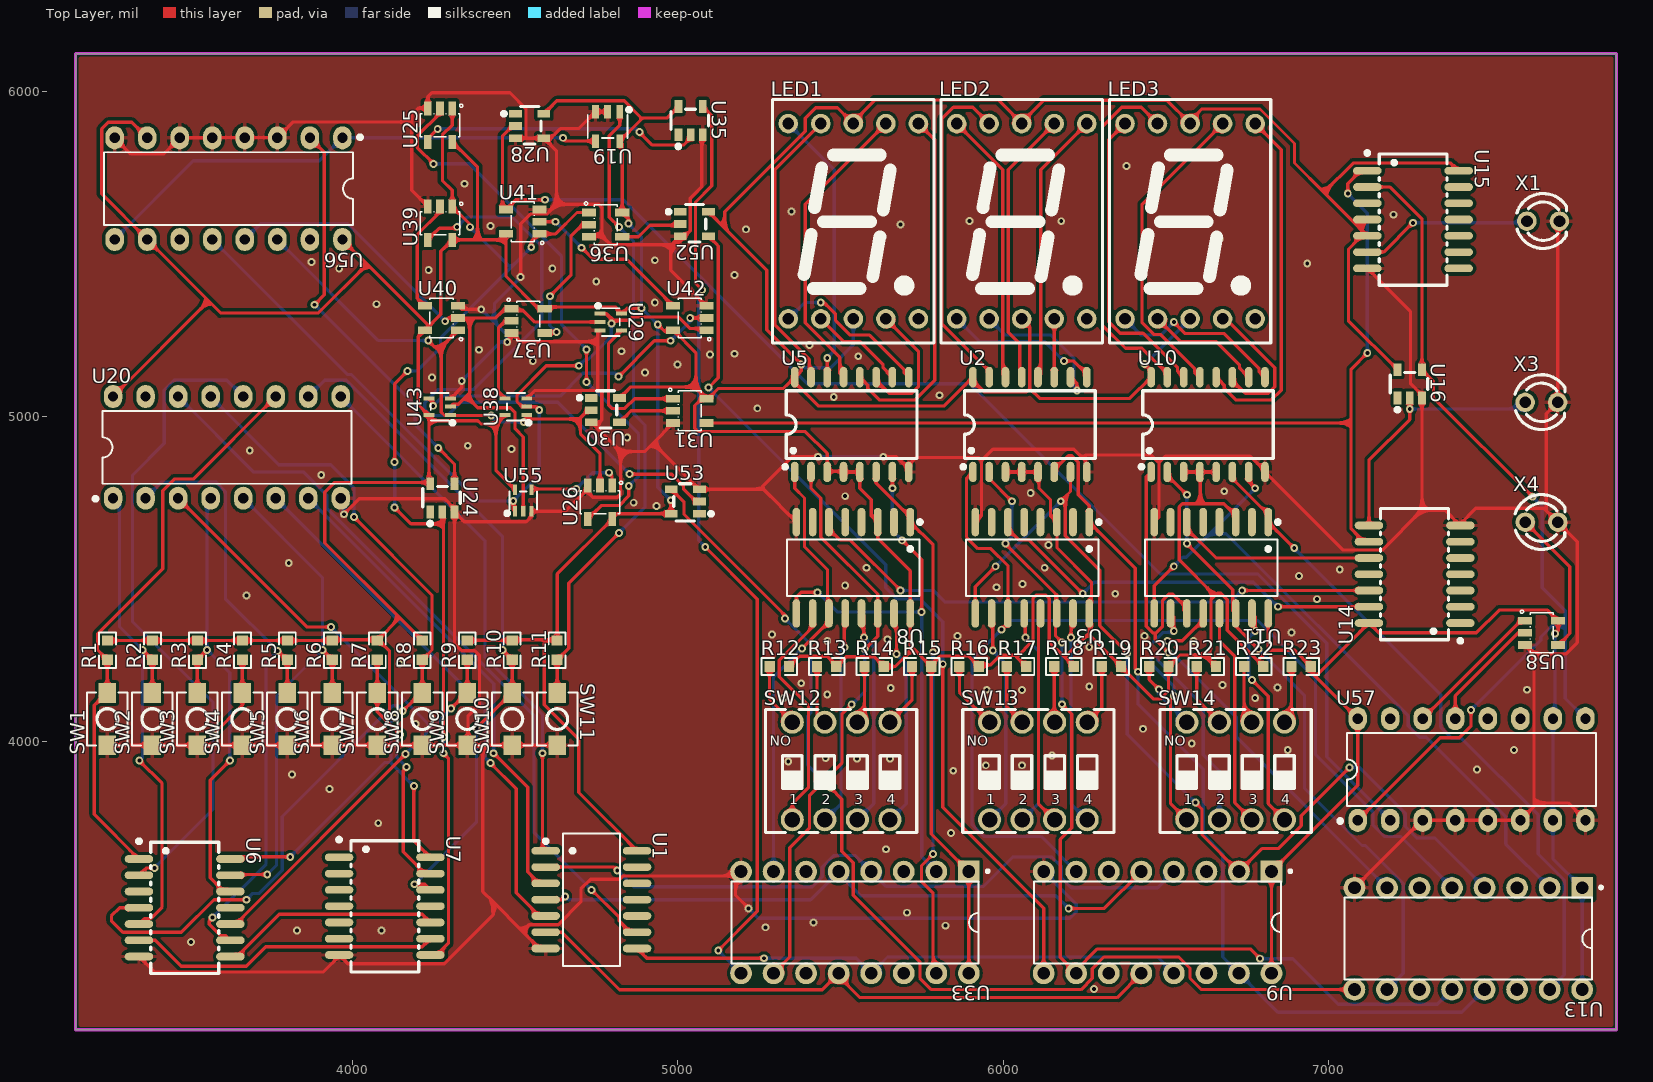
[diagram p0: Top Layer view]
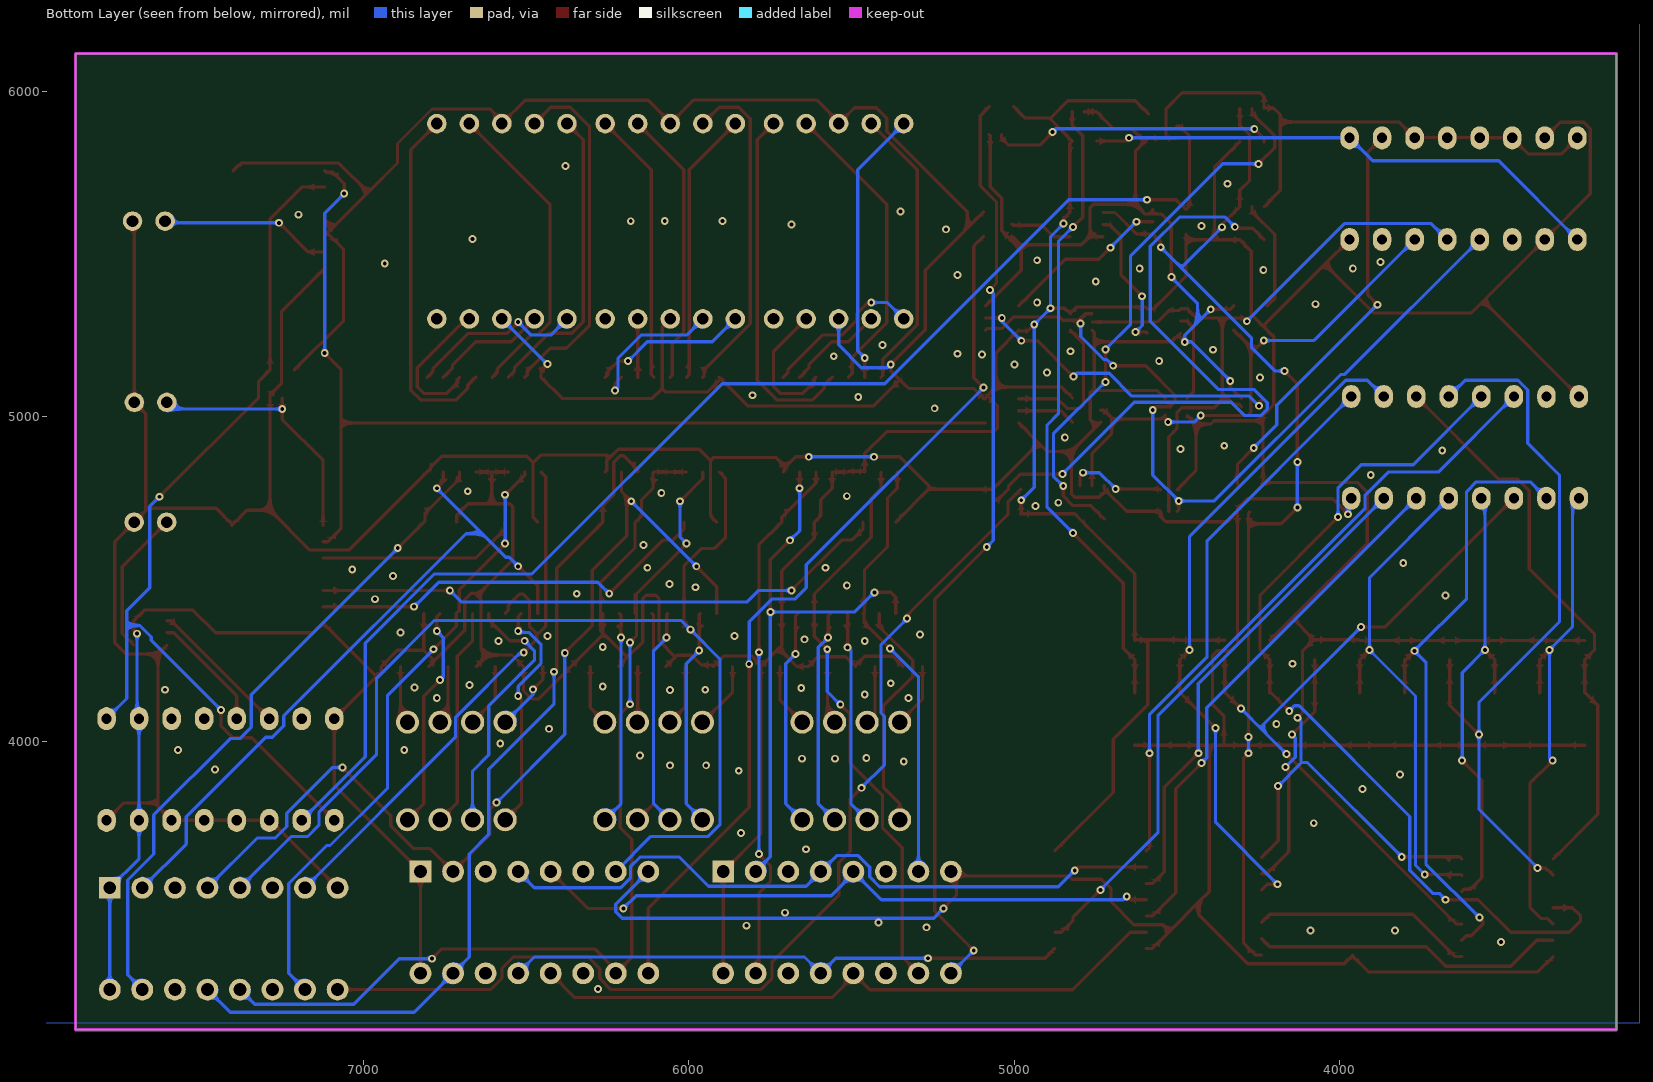
[diagram p1: Bottom Layer view, seen from below]
# Altium PCB MISC50897.pcbdoc (part 1 of 2)
Units mil, origin at the board's own origin, x right, y up, seen from the top; angles counter-clockwise.
Board outline 4735 x 3000 mil, 2 copper layers (Top Layer, Bottom Layer), stack 62.206 mil thick; 82 components, 112 nets, 500 pads, 251 vias.

## Layer stack, top to bottom
Top Solder Mask Layer: solder mask 0.394, Dk 3.3
Top Layer: signal copper 1.379
Dielectric1: surface 59.449, FR4, Dk 4.5
Bottom Layer: signal copper 1.378
Bottom Solder Mask Layer: solder mask 0.394, Dk 3.3

## Board outline
3150,6115 3150,3115 7885,3115 7885,6115

## Design rules (kind name [scope] priority, off if disabled: settings)
BoardOutlineClearance copperThickness2oz_1 [All] p2 off: genericclearance=7.99 ignorepadtopadclearanceinfootprint=FALSE except(0: Arc-SplitContinuation Track-SplitContinuation SMDPad-SplitContinuation THPad-SplitContinuation Via-SplitContinuation Fill-SplitContinuation Region-SplitContinuation Poly-SplitContinuation Text-SplitContinuation Hole-SplitContinuation; 5.98: Arc-CutoutEdge Track-CutoutEdge SMDPad-CutoutEdge THPad-CutoutEdge Via-CutoutEdge Text-CutoutEdge; 6.9: Hole-OutlineEdge Hole-CutoutEdge; 10: Poly-OutlineEdge Poly-CutoutEdge; 11.81: Arc-OutlineEdge Track-OutlineEdge SMDPad-OutlineEdge THPad-OutlineEdge Via-OutlineEdge Fill-OutlineEdge Region-OutlineEdge Text-OutlineEdge Fill-CutoutEdge Region-CutoutEdge)
BoardOutlineClearance Plane_innerPlane_1 [All] p4 off: genericclearance=4.02 ignorepadtopadclearanceinfootprint=FALSE except(0: Arc-SplitContinuation Track-SplitContinuation SMDPad-SplitContinuation THPad-SplitContinuation Via-SplitContinuation Fill-SplitContinuation Region-SplitContinuation Poly-SplitContinuation Text-SplitContinuation Hole-SplitContinuation; 5.98: Arc-CutoutEdge Track-CutoutEdge SMDPad-CutoutEdge THPad-CutoutEdge Via-CutoutEdge Text-CutoutEdge; 6.9: Hole-OutlineEdge Hole-CutoutEdge; 10: Poly-OutlineEdge Poly-CutoutEdge; 11.81: Arc-OutlineEdge Track-OutlineEdge SMDPad-OutlineEdge THPad-OutlineEdge Via-OutlineEdge Fill-OutlineEdge Region-OutlineEdge Text-OutlineEdge Fill-CutoutEdge Region-CutoutEdge)
BoardOutlineClearance Copper_copperRegion_1 [All] p6 off: genericclearance=4.02 ignorepadtopadclearanceinfootprint=FALSE except(0: Arc-SplitContinuation Track-SplitContinuation SMDPad-SplitContinuation THPad-SplitContinuation Via-SplitContinuation Fill-SplitContinuation Region-SplitContinuation Poly-SplitContinuation Text-SplitContinuation Hole-SplitContinuation; 5.98: Arc-CutoutEdge Track-CutoutEdge SMDPad-CutoutEdge THPad-CutoutEdge Via-CutoutEdge Text-CutoutEdge; 6.9: Hole-OutlineEdge Hole-CutoutEdge; 10: Poly-OutlineEdge Poly-CutoutEdge; 11.81: Arc-OutlineEdge Track-OutlineEdge SMDPad-OutlineEdge THPad-OutlineEdge Via-OutlineEdge Fill-OutlineEdge Region-OutlineEdge Text-OutlineEdge Fill-CutoutEdge Region-CutoutEdge)
BoardOutlineClearance copperThickness1oz_1 [All] p8: genericclearance=4.02 ignorepadtopadclearanceinfootprint=FALSE except(0: Arc-SplitContinuation Track-SplitContinuation SMDPad-SplitContinuation THPad-SplitContinuation Via-SplitContinuation Fill-SplitContinuation Region-SplitContinuation Poly-SplitContinuation Text-SplitContinuation Hole-SplitContinuation; 5.98: Arc-CutoutEdge Track-CutoutEdge SMDPad-CutoutEdge THPad-CutoutEdge Via-CutoutEdge Text-CutoutEdge; 6.9: Hole-OutlineEdge Hole-CutoutEdge; 10: Poly-OutlineEdge Poly-CutoutEdge; 11.81: Arc-OutlineEdge Track-OutlineEdge SMDPad-OutlineEdge THPad-OutlineEdge Via-OutlineEdge Fill-OutlineEdge Region-OutlineEdge Text-OutlineEdge Fill-CutoutEdge Region-CutoutEdge)
Clearance copperThickness2oz [All] p1 off: gap=7.99 ignorepadtopadclearanceinfootprint=FALSE except(5.98: SMDPad-Track SMDPad-SMDPad THPad-Track SMDPad-THPad THPad-THPad Track-Via SMDPad-Via THPad-Via Via-Via Fill-SMDPad Region-SMDPad Fill-THPad Region-THPad Fill-Via Region-Via Fill-Fill Fill-Region Region-Region Arc-Track Arc-SMDPad Arc-THPad Arc-Via Fill-Arc Region-Arc Arc-Arc Text-Track SMDPad-Text Text-THPad Text-Via Fill-Text Region-Text Arc-Text Text-Text; 6.9: Hole-Track Hole-SMDPad Hole-THPad Hole-Via Fill-Hole Region-Hole Hole-Arc Hole-Text; 10: Poly-Track Poly-SMDPad Poly-THPad Poly-Via Poly-Fill Poly-Region Poly-Poly Poly-Arc Poly-Text Poly-Hole; 11.81: Fill-Track Region-Track)
Clearance Plane_innerPlane [All] p3 off: gap=4.02 ignorepadtopadclearanceinfootprint=FALSE except(5.98: SMDPad-Track SMDPad-SMDPad THPad-Track SMDPad-THPad THPad-THPad Track-Via SMDPad-Via THPad-Via Via-Via Fill-SMDPad Region-SMDPad Fill-THPad Region-THPad Fill-Via Region-Via Fill-Fill Fill-Region Region-Region Arc-Track Arc-SMDPad Arc-THPad Arc-Via Fill-Arc Region-Arc Arc-Arc Text-Track SMDPad-Text Text-THPad Text-Via Fill-Text Region-Text Arc-Text Text-Text; 6.9: Hole-Track Hole-SMDPad Hole-THPad Hole-Via Fill-Hole Region-Hole Hole-Arc Hole-Text; 10: Poly-Track Poly-SMDPad Poly-THPad Poly-Via Poly-Fill Poly-Region Poly-Poly Poly-Arc Poly-Text Poly-Hole; 11.81: Fill-Track Region-Track)
Clearance Copper_copperRegion [All] p5 off: gap=4.02 ignorepadtopadclearanceinfootprint=FALSE except(5.98: SMDPad-Track SMDPad-SMDPad THPad-Track SMDPad-THPad THPad-THPad Track-Via SMDPad-Via THPad-Via Via-Via Fill-SMDPad Region-SMDPad Fill-THPad Region-THPad Fill-Via Region-Via Fill-Fill Fill-Region Region-Region Arc-Track Arc-SMDPad Arc-THPad Arc-Via Fill-Arc Region-Arc Arc-Arc Text-Track SMDPad-Text Text-THPad Text-Via Fill-Text Region-Text Arc-Text Text-Text; 6.9: Hole-Track Hole-SMDPad Hole-THPad Hole-Via Fill-Hole Region-Hole Hole-Arc Hole-Text; 10: Poly-Track Poly-SMDPad Poly-THPad Poly-Via Poly-Fill Poly-Region Poly-Poly Poly-Arc Poly-Text Poly-Hole; 11.81: Fill-Track Region-Track)
Clearance copperThickness1oz [All] p7: gap=4.02 ignorepadtopadclearanceinfootprint=FALSE except(5.98: SMDPad-Track SMDPad-SMDPad THPad-Track SMDPad-THPad THPad-THPad Track-Via SMDPad-Via THPad-Via Via-Via Fill-SMDPad Region-SMDPad Fill-THPad Region-THPad Fill-Via Region-Via Fill-Fill Fill-Region Region-Region Arc-Track Arc-SMDPad Arc-THPad Arc-Via Fill-Arc Region-Arc Arc-Arc Text-Track SMDPad-Text Text-THPad Text-Via Fill-Text Region-Text Arc-Text Text-Text; 6.9: Hole-Track Hole-SMDPad Hole-THPad Hole-Via Fill-Hole Region-Hole Hole-Arc Hole-Text; 10: Poly-Track Poly-SMDPad Poly-THPad Poly-Via Poly-Fill Poly-Region Poly-Poly Poly-Arc Poly-Text Poly-Hole; 11.81: Fill-Track Region-Track)
DiffPairsRouting differentialPair [All] p1: maxlimit=6 minlimit=6 mostfreqgap=6 toplayer_minwidth=5 toplayer_prefwidth=10 toplayer_maxwidth=100 toplayer_mingap=6 toplayer_prefgap=6 toplayer_maxgap=6 bottomlayer_minwidth=5 bottomlayer_prefwidth=10 bottomlayer_maxwidth=100 bottomlayer_mingap=6 bottomlayer_prefgap=6 bottomlayer_maxgap=6 maxuncoupledlength=10
HoleToHoleClearance otherClearance [All] p1: gap=11.81 allowstackedmicrovias=TRUE
Length netLength [All] p1: minlimit=0 maxlimit=0
PasteMaskExpansion pasteMaskExpansion [All] p1: expansion=0
PlaneConnect innerPlane [All] p1: planeconnectstyle=Relief reliefexpansion=20 reliefentries=4 reliefconductorwidth=10 reliefairgap=10
PolygonConnect copperRegion [All] p1: connectstyle=Relief reliefconductorwidth=10 reliefentries=4 polygonreliefangle="90 Angle" airgapwidth=10 via.connectstyle=Relief via.reliefconductorwidth=10 via.reliefentries=4 via.polygonreliefangle="90 Angle" via.airgapwidth=10
RoutingVias viaSize [All] p1: holewidth=12.01 width=24.02 viastyle="Through Hole" minholewidth=11.81 minwidth=19.68 maxholewidth=248.03 maxwidth=393.7
SolderMaskExpansion solderMaskExpansion [IsVia] p1: expansion=-1000 istentingtop=TRUE
SolderMaskExpansion solderMaskExpansion [All] p2: expansion=2 istentingtop=FALSE
Width copperThickness2oz_2 [All] p1 off: maxlimit=100 minlimit=8 preferedwidth=10
Width copperThickness1oz_2 [All] p2: maxlimit=100 minlimit=5 preferedwidth=10

## Components (designator, comment, footprint, x,y, rotation, side; value= is the part's Value field where it differs from the comment)
LED1 "" LED-SEG-TH_10P-L12.6-W19.0-P2.54-S15.24-BL 5540,5600 r0 top
LED2 "" LED-SEG-TH_10P-L12.6-W19.0-P2.54-S15.24-BL 6057.5,5600 r0 top
LED3 "" LED-SEG-TH_10P-L12.6-W19.0-P2.54-S15.24-BL 6575,5600 r0 top
R1 "1K" R0603 3247.53,4281.89 r90 top
R2 "1K" R0603 3385.78,4281.89 r90 top
R3 "1K" R0603 3524.02,4281.89 r90 top
R4 "1K" R0603 3662.27,4281.89 r90 top
R5 "1K" R0603 3800.52,4281.89 r90 top
R6 "1K" R0603 3938.77,4281.89 r90 top
R7 "1K" R0603 4077.01,4281.89 r90 top
R8 "1K" R0603 4215.26,4281.89 r90 top
R9 "1K" R0603 4353.51,4281.89 r90 top
R10 "1K" R0603 4491.75,4281.89 r90 top
R11 "1K" R0603 4630,4281.89 r90 top
R12 "1K" R0603 5312.43,4231.43 r0 top
R13 "1K" R0603 5458.25,4231.43 r0 top
R14 "1K" R0603 5604.06,4231.43 r0 top
R15 "1K" R0603 5749.88,4231.43 r0 top
R16 "1K" R0603 5895.7,4231.43 r0 top
R17 "1K" R0603 6041.52,4231.43 r0 top
R18 "1K" R0603 6187.34,4231.43 r0 top
R19 "1K" R0603 6333.15,4231.43 r0 top
R20 "1K" R0603 6478.97,4231.43 r0 top
R21 "1K" R0603 6624.79,4231.43 r0 top
R22 "1K" R0603 6770.61,4231.43 r0 top
R23 "1K" R0603 6916.43,4231.43 r0 top
SW1 "轻触按键3*4*H" SW-SMD_L4.0-W2.9-LS5.0 3247.53,4070 r90 top
SW2 "轻触按键3*4*H" SW-SMD_L4.0-W2.9-LS5.0 3385.78,4070 r90 top
SW3 "轻触按键3*4*H" SW-SMD_L4.0-W2.9-LS5.0 3524.02,4070 r90 top
SW4 "轻触按键3*4*H" SW-SMD_L4.0-W2.9-LS5.0 3662.27,4070 r90 top
SW5 "轻触按键3*4*H" SW-SMD_L4.0-W2.9-LS5.0 3800.52,4070 r90 top
SW6 "轻触按键3*4*H" SW-SMD_L4.0-W2.9-LS5.0 3938.77,4070 r90 top
SW7 "轻触按键3*4*H" SW-SMD_L4.0-W2.9-LS5.0 4077.01,4070 r90 top
SW8 "轻触按键3*4*H" SW-SMD_L4.0-W2.9-LS5.0 4215.26,4070 r90 top
SW9 "轻触按键3*4*H" SW-SMD_L4.0-W2.9-LS5.0 4353.51,4070 r90 top
SW10 "轻触按键3*4*H" SW-SMD_L4.0-W2.9-LS5.0 4491.75,4070 r90 top
SW11 "轻触按键3*4*H" SW-SMD_L4.0-W2.9-LS5.0 4630,4070 r270 top
SW12 "DSWB04LHGET" SW-TH_DSWB04LHGET 5502.43,3910.4 r0 top
SW13 "DSWB04LHGET" SW-TH_DSWB04LHGET 6108.71,3910.4 r0 top
SW14 "DSWB04LHGET" SW-TH_DSWB04LHGET 6715,3910.4 r0 top
U1 "SN74LS04NSR" SOIC-14_L10.0-W5.5-P1.27-LS7.8-BL 4735,3515 r270 top
U2 "SN74LS47NSR" SO-16_L10.2-W5.3-P1.27-LS7.8-BL 6082.5,4975 r0 top
U3 "SN74LS85NS" SOIC-16_L10.8-W5.5-P1.27-LS7.8-BL 6090,4535 r180 top
U5 "SN74LS47NSR" SO-16_L10.2-W5.3-P1.27-LS7.8-BL 5535,4975 r0 top
U6 "SN74HC21NSR" SO-14_L10.2-W5.3-P1.27-LS7.8-BL-1 3485,3490 r270 top
U7 "SN74HC21NSR" SO-14_L10.2-W5.3-P1.27-LS7.8-BL-1 4100,3495 r270 top
U8 "SN74LS85NS" SOIC-16_L10.8-W5.5-P1.27-LS7.8-BL 5540,4535 r180 top
U9 "SN74S175N" PDIP-16_L19.3-W6.4-P2.54-LS7.9-BL 6475,3445 r180 top
U10 "SN74LS47NSR" SO-16_L10.2-W5.3-P1.27-LS7.8-BL 6630,4975 r0 top
U11 "SN74LS85NS" SOIC-16_L10.8-W5.5-P1.27-LS7.8-BL 6640,4535 r180 top
U13 "SN74S175N" PDIP-16_L19.3-W6.4-P2.54-LS7.9-BL 7430,3395 r180 top
U14 "SN74HC21NSR" SO-14_L10.2-W5.3-P1.27-LS7.8-BL-1 7265,4515 r90 top
U15 "SN74HC21NSR" SO-14_L10.2-W5.3-P1.27-LS7.8-BL-1 7260,5605 r270 top
U16 "NC7SU04M5-FS" SOT-23-5_L2.9-W1.6-P0.95-LS2.8-BR 7250,5100 r270 top
U19 "NC7S08M5" SOT-23-5_L3.0-W1.5-P0.95-LS2.8-BL 4785,5891.44 r180 top
U20 "SN74LS147N(LX)" PDIP-16_L19.3-W6.4-P2.54-LS7.94-BL 3615,4905 r0 top
U24 "NC7SU04M5-FS" SOT-23-5_L2.9-W1.6-P0.95-LS2.8-BR 4276.99,4750 r270 top
U25 "NC7S08M5X" SOT-23-5_L3.0-W1.7-P0.95-LS2.8-BR 4270,5895 r90 top
U26 "NC7S08M5X" SOT-23-5_L3.0-W1.7-P0.95-LS2.8-BR 4761.29,4736.03 r90 top
U28 "NC7SU04M5-FS" SOT-23-5_L2.9-W1.6-P0.95-LS2.8-BR 4545.42,5892.5 r180 top
U29 "NC7S02P5X" SC-70-5_L2.1-W1.3-P0.65-LS2.1-BL 4794.59,5290.11 r270 top
U30 "NC7SU04M5-FS" SOT-23-5_L2.9-W1.6-P0.95-LS2.8-BR 4778.05,5019.32 r180 top
U31 "NC7S08M5X" SOT-23-5_L3.0-W1.7-P0.95-LS2.8-BR 5037.5,5017.34 r180 top
U33 "SN74S175N" PDIP-16_L19.3-W6.4-P2.54-LS7.9-BL 5545,3445 r180 top
U35 "NC7SU04M5-FS" SOT-23-5_L2.9-W1.6-P0.95-LS2.8-BR 5040,5908.97 r270 top
U36 "NC7S08M5X" SOT-23-5_L3.0-W1.7-P0.95-LS2.8-BR 4778.62,5589.4 r180 top
U37 "NC7S08M5X" SOT-23-5_L3.0-W1.7-P0.95-LS2.8-BR 4540.63,5293.64 r180 top
U38 "NC7S02P5X" SC-70-5_L2.1-W1.3-P0.65-LS2.1-BL 4502.83,5029.85 r90 top
U39 "NC7S08M5X" SOT-23-5_L3.0-W1.7-P0.95-LS2.8-BR 4270,5593.89 r90 top
U40 "NC7S08M5X" SOT-23-5_L3.0-W1.7-P0.95-LS2.8-BR 4274.49,5302.62 r0 top
U41 "NC7S08M5X" SOT-23-5_L3.0-W1.7-P0.95-LS2.8-BR 4523.88,5598.38 r0 top
U42 "NC7S08M5X" SOT-23-5_L3.0-W1.7-P0.95-LS2.8-BR 5037.5,5302.62 r0 top
U43 "NC7S02P5X" SC-70-5_L2.1-W1.3-P0.65-LS2.1-BL 4268.96,5029.85 r90 top
U52 "NC7SU04M5-FS" SOT-23-5_L2.9-W1.6-P0.95-LS2.8-BR 5051.47,5591.39 r180 top
U53 "NC7SU04M5-FS" SOT-23-5_L2.9-W1.6-P0.95-LS2.8-BR 5023.53,4738.53 r0 top
U55 "NC7S02P5X" SC-70-5_L2.1-W1.3-P0.65-LS2.1-BL 4525.67,4741.56 r0 top
U56 "SN74LS161N(LX)" PDIP-16_L19.3-W6.4-P2.54-LS7.94-BL 3620,5700 r180 top
U57 "SN74LS161N(LX)" PDIP-16_L19.3-W6.4-P2.54-LS7.94-BL 7440,3915 r0 top
U58 "NC7S08M5X" SOT-23-5_L3.0-W1.7-P0.95-LS2.8-BR 7655,4335 r180 top
X1 "" LED_TH-3mm 7660,5600 r0 top
X3 "" LED_TH-3mm 7654.69,5043.42 r0 top
X4 "" LED_TH-3mm 7655,4675 r0 top

## Footprints (in the part's own frame and the unit in brackets; to place one, negate y for a bottom-side part, rotate by r counter-clockwise, add the part's x,y. Pads: shape width x height; smd on the part's side, far side on the other; paste and mask are expansions set on the pad)
LED-SEG-TH_10P-L12.6-W19.0-P2.54-S15.24-BL [mil]
  round 60 hole 36: 1(-200,-300) 2(-100,-300) 3(0,-300) 4(100,-300) 5(200,-300) 6(200,300) 7(100,300) 8(0,300) 9(-100,300) 10(-200,300)
  silkscreen extent -248,-374 248,374
LED_TH-3mm [mil]
  round 60 hole 36 paste+0 mask+2: 1(-50,0) 2(50,0)
  silkscreen extent -81,-84 72,85
PDIP-16_L19.3-W6.4-P2.54-LS7.9-BL [mm]
  rect 1.7x1.7 hole 1: 1(-8.89,-3.97)
  round 1.7 hole 1 copper offset 0,0: 2(-6.35,-3.97) 3(-3.81,-3.97) 4(-1.27,-3.97) 5(1.27,-3.97) 6(3.81,-3.97) 7(6.35,-3.97) 8(8.89,-3.97)
  round 1.7 hole 1: 9(8.89,3.97) 10(6.35,3.97) 11(3.81,3.97) 12(1.27,3.97) 13(-1.27,3.97) 14(-3.81,3.97) 15(-6.35,3.97) 16(-8.89,3.97)
  silkscreen extent -10.46,-4.1 9.65,3.2
PDIP-16_L19.3-W6.4-P2.54-LS7.94-BL [mm]
  oval 1.44x1.8 hole 0.8: 1(-8.89,-3.97) 2(-6.35,-3.97) 3(-3.81,-3.97) 4(-1.27,-3.97) 5(1.27,-3.97) 6(3.81,-3.97) 7(6.35,-3.97) 8(8.89,-3.97) 9(8.89,3.97) 10(6.35,3.97) 11(3.81,3.97) 12(1.27,3.97) 13(-1.27,3.97) 14(-3.81,3.97) 15(-6.35,3.97) 16(-8.89,3.97)
  silkscreen extent -10.41,-4.17 9.73,2.84
R0603 [mil]
  rect 31.75x34.02 smd paste-3937.01 mask+2: 1(-29.66,0) 2(29.66,0)
  silkscreen extent -55,-26 55,26
SC-70-5_L2.1-W1.3-P0.65-LS2.1-BL [mm]
  rect 0.315x0.835 smd: 1(-0.65,-0.843) 2(0,-0.843) 3(0.65,-0.843) 4(0.65,0.842) 5(-0.65,0.842)
  silkscreen extent -1.41,-1.14 1.08,0.7
SO-14_L10.2-W5.3-P1.27-LS7.8-BL-1 [mil]
  oval 23.7x87.83 smd: 1(-150,-140.37) 2(-100,-140.37) 3(-50,-140.37) 4(0,-140.37) 5(50,-140.37) 6(100,-140.37) 7(150,-140.37) 8(150,140.37) 9(100,140.37) 10(50,140.37) 11(0,140.37) 12(-50,140.37) 13(-100,140.37) 14(-150,140.37)
  silkscreen extent -211,-146 202,105
SO-16_L10.2-W5.3-P1.27-LS7.8-BL [mil]
  oval 23.43x62.89 smd: 1(-175,-145.67) 2(-125,-145.67) 3(-75,-145.67) 4(-25,-145.67) 5(25,-145.67) 6(75,-145.67) 7(125,-145.67) 8(175,-145.67) 9(175,145.67) 10(125,145.67) 11(75,145.67) 12(25,145.67) 13(-25,145.67) 14(-75,145.67) 15(-125,145.67) 16(-175,145.67)
  silkscreen extent -210,-136 201,104
SOIC-14_L10.0-W5.5-P1.27-LS7.8-BL [mil]
  oval 23.7x87.83 smd: 1(-150,-140.37) 2(-100,-140.37) 3(-50,-140.37) 4(0,-140.37) 5(50,-140.37) 6(100,-140.37) 7(150,-140.37) 8(150,140.37) 9(100,140.37) 10(50,140.37) 11(0,140.37) 12(-50,140.37) 13(-100,140.37) 14(-150,140.37)
  silkscreen extent -204,-146 204,87
SOIC-16_L10.8-W5.5-P1.27-LS7.8-BL [mil]
  oval 23.7x87.83 smd: 1(-175,-140.37) 2(-125,-140.37) 3(-75,-140.37) 4(-25,-140.37) 5(25,-140.37) 6(75,-140.37) 7(125,-140.37) 8(175,-140.37) 9(175,140.37) 10(125,140.37) 11(75,140.37) 12(25,140.37) 13(-25,140.37) 14(-75,140.37) 15(-125,140.37) 16(-175,140.37)
  silkscreen extent -211,-146 204,87
SOT-23-5_L2.9-W1.6-P0.95-LS2.8-BR [mm]
  rect 1x0.6 smd paste+0 mask+0.05: 1(1.1,-0.95) 2(1.1,0) 3(1.1,0.95) 4(-1.1,0.95) 5(-1.1,-0.95)
  silkscreen extent -0.89,-1.52 2.16,1.4
SOT-23-5_L3.0-W1.5-P0.95-LS2.8-BL [mm]
  rect 0.532x1.045 smd: 1(-0.95,-1.148) 2(0,-1.148) 3(0.95,-1.148) 4(0.95,1.148) 5(-0.95,1.148)
  silkscreen extent -1.82,-1.45 1.55,0.9
SOT-23-5_L3.0-W1.7-P0.95-LS2.8-BR [mm]
  rect 1.1x0.6 smd: 1(1.3,-0.95) 2(1.3,0) 3(1.3,0.95) 4(-1.3,0.95) 5(-1.3,-0.95)
  silkscreen extent -0.9,-1.78 1.65,1.55
SW-SMD_L4.0-W2.9-LS5.0 [mm]
  rect 1.53x1.36 smd: 1(-2.035,0) 2(2.035,0)
  silkscreen extent -2.08,-1.58 2.08,1.58
SW-TH_DSWB04LHGET [mm]
  round 1.8 hole 1.2: 1(-3.81,3.81) 2(-1.27,3.81) 3(1.27,3.81) 4(3.81,3.81) 5(-3.81,-3.81) 6(-1.27,-3.81) 7(1.27,-3.81) 8(3.81,-3.81)
  silkscreen extent -5.9,-4.8 5.9,4.8

## Via types
v1: diameter 24.02, hole 12, Top Layer to Bottom Layer, 251 vias

## Nets (pads, with @x,y where several pads share a name; then routed paths per layer and width w, separated by ;. In a path a pad name is that pad's centre, name@x,y a point inside that pad or via, vN(x,y) a via of type N, cw(c..) or ccw(c..) an arc to the next point about the centre after c; other vN are vias at no path point)
$1N1634: R1.1 SW1.2 U6.1 U20.11 | length 1770.2
  Top Layer w10: SW1.2@3247.53,4150.12 SW1.2@3247.53,4152.23 ; U6.1@3344.63,3640 3207.53,3777.1 3207.53,4112.23 SW1.2@3247.53,4152.23 ; U20.11@3765,5061.3 3511.29,4807.59 3452.89,4807.59 3417.53,4772.23 3417.53,4532.23 3217.53,4332.23 3217.53,4282.23 R1.1@3247.53,4252.23 SW1.2@3247.53,4152.23
$1N1649: R3.1 SW3.2 U6.12 U20.4 | length 1448.2
  Top Layer w10: SW3.2@3524.02,4150.12 R3.1@3524.02,4252.23 v1(3554.02,4282.23) ; v1(3624.02,3942.23) 3564.02,3882.23 3564.02,3582.23 3599.38,3546.87 3618.5,3546.87 U6.12@3625.37,3540
  Bottom Layer w10: U20.4@3565,4748.7 3554.02,4737.72 v1(3554.02,4282.23) 3624.02,4212.23 v1(3624.02,3942.23)
$1N1673: R5.1 SW5.2 U6.9 U20.2 | length 1990.9
  Top Layer w10: v1(3570.52,3459.73) 3560.52,3449.73 3560.52,3439.73 3595.87,3404.37 3611,3404.37 U6.9@3625.37,3390 ; v1(3770.52,4279.73) R5.1@3800.52,4249.73 ; SW5.2@3800.52,4150.12 R5.1@3800.52,4249.73 ; R5.1@3800.52,4252.23 R5.1@3800.52,4249.73
  Bottom Layer w10: U20.2@3365,4748.7 3415,4798.7 3580.52,4798.7 3610.52,4768.7 3610.52,4439.73 v1(3770.52,4279.73) 3735.16,4244.37 3735.16,3624.37 v1(3570.52,3459.73)
$1N1683: R4.1 SW4.2 U6.2 U20.12 | length 2286.5
  Top Layer w10: U6.2@3344.63,3590 3366.86,3612.23 v1(3392.27,3612.23) ; v1(3572.27,4022.23) 3662.27,4112.23 R4.1@3662.27,4252.23
  Bottom Layer w10: v1(3392.27,3612.23) 3572.27,3792.23 v1(3572.27,4022.23) 3572.27,4122.23 3324.78,4369.72 3324.78,4819.72 3422.27,4917.2 3422.27,5081.3 3452.27,5111.3 3615,5111.3 U20.12@3665,5061.3
$1N1696: R2.1 SW2.2 U6.5 U20.1 | length 1564.5
  Top Layer w10: U6.5@3344.63,3440 3361.5,3456.87 3380.42,3456.87 3415.78,3492.23 3415.78,3872.23 v1(3345.78,3942.23) ; v1(3355.78,4282.23) R2.1@3385.78,4252.23 SW2.2@3385.78,4150.12
  Bottom Layer w10: U20.1@3265,4748.7 3285.07,4728.63 3285.07,4352.94 v1(3355.78,4282.23) 3355.78,3952.23 v1(3345.78,3942.23)
$1N1728: R6.1 SW6.2 U6.13 U20.5 | length 1586.7
  Top Layer w10: U6.13@3625.37,3590 3627.6,3592.23 v1(3738.77,3592.23) ; v1(3908.77,4282.23) R6.1@3938.77,4252.23 SW6.2@3938.77,4150.12
  Bottom Layer w10: U20.5@3665,4748.7 3908.77,4504.93 v1(3908.77,4282.23) 3767.34,4140.81 3767.34,3620.81 v1(3738.77,3592.23)
$1N1735: R7.1 SW7.2 U7.13 | length 750.9
  Top Layer w10: R7.1@4077.01,4252.23 4077.01,4092.23 v1(4147.01,4022.23) ; v1(4167.01,3922.23) 4157.01,3912.23 4157.01,3662.23 4224.24,3595 U7.13@4240.37,3595
  Bottom Layer w10: v1(4147.01,4022.23) 4137.01,4012.23 4137.01,3952.23 v1(4167.01,3922.23)
$1N1743: R8.1 SW8.2 U6.4 U20.13 | length 2795.8
  Top Layer w10: U6.4@3344.63,3490 3285,3490 3260,3465 3260,3450 3295.27,3414.73 3475.26,3414.73 3575.26,3514.73 v1(3675.26,3514.73) ; v1(4005.26,4691.04) 4245.26,4451.04 4245.26,4282.23 R8.1@4215.26,4252.23 SW8.2@4215.26,4154.73 ; v1(4155.26,4094.73) SW8.2@4215.26,4154.73 ; SW8.2@4215.26,4150.12 SW8.2@4215.26,4154.73
  Bottom Layer w10: U20.13@3565,5061.3 3774.55,4851.75 3934.55,4851.75 4005.26,4781.04 v1(4005.26,4691.04) ; v1(3675.26,3514.73) 3694.55,3534.02 3714.55,3534.02 3785.26,3604.73 3785.26,3770.59 4125.26,4110.59 4139.4,4110.59 v1(4155.26,4094.73)
$1N1750: R9.1 SW9.2 U6.10 U20.3 | length 2202.9
  Top Layer w10: U20.3@3465,4748.7 3860.41,4353.29 v1(3934.56,4353.29) ; U6.10@3625.37,3440 3641.28,3440 v1(4163.51,3962.23) ; v1(4303.51,4102.23) SW9.2@4353.51,4152.23 ; SW9.2@4353.51,4150.12 SW9.2@4353.51,4152.23 ; R9.1@4353.51,4252.23 SW9.2@4353.51,4152.23
  Bottom Layer w10: v1(3934.56,4353.29) 4234.56,4053.29 4234.56,4033.29 ; v1(4163.51,3962.23) 4234.56,4033.29 ; v1(4303.51,4102.23) 4234.56,4033.29
$1N1758: R10.1 SW10.2 U7.12 U20.10 | length 2079.9
  Top Layer w10: v1(4191.75,3562.23) 4223.14,3562.23 U7.12@4240.37,3545 ; v1(4381.75,4042.23) SW10.2@4491.75,4152.23 ; v1(4461.75,4282.23) R10.1@4491.75,4252.23 SW10.2@4491.75,4152.23 ; SW10.2@4491.75,4150.12 SW10.2@4491.75,4152.23
  Bottom Layer w10: U20.10@3865,5061.3 3915,5111.3 3981.75,5111.3 4461.75,4631.3 v1(4461.75,4282.23) ; v1(4191.75,3562.23) 4381.75,3752.23 v1(4381.75,4042.23)
$1N2590: U6.6 U7.9 | length 964.1
  Top Layer w10: U6.6@3344.63,3390 3394.63,3390 3474.63,3310 3674.63,3310 3734.63,3370 4215.37,3370 U7.9@4240.37,3395
$1N2596: U6.8 U7.10 | length 679.2
  Top Layer w10: U6.8@3625.37,3340 3645.37,3340 3775.37,3470 4215.37,3470 U7.10@4240.37,3445
$1N2812: R11.1 SW11.1 U19.1 | length 1957.3
  Top Layer w10: SW11.1@4630,4150.12 R11.1@4630,4252.23 4665.36,4287.59 4665.36,4487.59 v1(4820,4642.23) ; v1(4820,5582.23) 4790,5612.23 4790,5862.23 4822.4,5894.63 U19.1@4822.4,5936.62
  Bottom Layer w10: v1(4820,4642.23) 4900,4722.23 4900,4972.23 4864.64,5007.59 4864.64,5537.59 v1(4820,5582.23)
$1N3570: U1.1 U20.9 | length 1657.1
  Top Layer w10: v1(4584.63,3965) 4584.63,3675 U1.1@4594.63,3665
  Bottom Layer w10: U20.9@3965,5061.3 4407.85,4618.45 4407.85,4261.78 4584.63,4085 v1(4584.63,3965)
$1N3574: U1.3 U20.7 | length 1497.6
  Top Layer w10: v1(4434.63,3965) 4539.27,3860.36 4539.27,3600.36 4574.63,3565 U1.3@4594.63,3565
  Bottom Layer w10: U20.7@3865,4748.7 4434.63,4179.07 v1(4434.63,3965)
$1N3581: U1.5 U20.6 | length 1639.1
  Top Layer w10: v1(4424.63,3935) 4503.92,3855.71 4503.92,3535.71 4574.63,3465 U1.5@4594.63,3465
  Bottom Layer w10: U20.6@3765,4748.7 4408.64,4105.06 4408.64,3950.99 v1(4424.63,3935)
$1N3588: U1.9 U20.14 | length 2332.5
  Top Layer w10: v1(4735.37,3545) 4820.01,3460.36 4820.01,3450.36 4855.37,3415 U1.9@4875.37,3415
  Bottom Layer w10: U20.14@3465,5061.3 3697.42,4828.88 3851.49,4828.88 3922.2,4758.17 3922.2,4718.17 4558.59,4081.78 4558.59,3721.78 v1(4735.37,3545)
$1N4417: U1.2 U9.4 U33.4 | length 2169
  Top Layer w10: U1.2@4594.63,3615 4804.63,3615 v1(4814.63,3605)
  Bottom Layer w10: v1(4814.63,3605) 4864.63,3555 5414.63,3555 5444.63,3585 5444.63,3615 5479.99,3650.36 5545.94,3650.36 U33.4@5594.99,3601.3 5640.14,3556.16 5940.14,3556.16 6030.14,3646.16 6150.14,3646.16 6180.14,3616.16 6180.14,3581.3 6210.14,3551.3 6475,3551.3 U9.4@6524.99,3601.3
$1N4426: U1.4 U9.5 U33.5 | length 1970.1
  Top Layer w10: U1.4@4594.63,3515 4644.63,3515 v1(4654.63,3525) ; v1(6201.78,3488.09) 6311.78,3488.09 U9.5@6424.99,3601.3
  Bottom Layer w10: v1(4654.63,3525) 4664.63,3515 5408.7,3515 U33.5@5491.78,3598.09 ; U33.5@5494.99,3601.3 U33.5@5491.78,3598.09 ; v1(6201.78,3488.09) 6162.5,3527.37 5562.5,3527.37 U33.5@5491.78,3598.09
$1N4432: U1.6 U9.12 U33.12 | length 1988.9
  Top Layer w10: U1.6@4594.63,3415 4644.63,3415 4821.41,3238.22 5444.52,3238.22 U33.12@5490.49,3284.19 ; U33.12@5495,3288.7 U33.12@5490.49,3284.19 ; U9.12@6425,3288.7 6350.49,3214.19 5560.49,3214.19 U33.12@5490.49,3284.19
$1N4439: U1.8 U9.13 U33.13 | length 1722.7
  Top Layer w10: U1.8@4875.37,3365 4905.37,3335 v1(5265.37,3335)
  Bottom Layer w10: v1(5265.37,3335) 5548.7,3335 U33.13@5595,3288.7 5645,3338.7 6475,3338.7 U9.13@6525,3288.7
$1N6186: LED1.1 U5.9 | length 502.9
  Top Layer w10: v1(5440,5350) 5450,5350 5485.36,5314.64 5485.36,5294.64 5530,5250 5590,5250 5696.07,5143.93 5696.07,5134.61 U5.9@5710,5120.67
  Bottom Layer w10: LED1.1@5340,5300 5390,5350 v1(5440,5350)
$1N6188: LED1.2 U5.10 | length 299.7
  Top Layer w10: LED1.2@5440,5300 5510.71,5229.29 5560.71,5229.29 5631.42,5158.58 5631.42,5149.25 U5.10@5660,5120.67
$1N6190: LED1.4 U5.11 | length 415.6
  Top Layer w10: U5.11@5610,5120.67 5614.65,5116.03 5614.65,5106.03 5650,5070.67 5720,5070.67 5740,5090.67 5740,5200 LED1.4@5640,5300
$1N6192: LED1.6 U5.12 | length 1099.7
  Top Layer w10: U5.12@5560,5120.67 5584.65,5096.03 5584.65,5086.03 5620,5050.67 5730,5050.67 5790,5110.67 5790,5850 LED1.6@5740,5900
$1N6194: LED1.7 U5.13 | length 930.5
  Top Layer w10: U5.13@5510,5120.67 5498.58,5132.09 5498.58,5181.42 5392.51,5287.49 5392.51,5652.51 LED1.7@5640,5900
$1N6196: LED1.10 U5.14 | length 846.8
  Top Layer w10: U5.14@5460,5120.67 v1(5460,5180)
  Bottom Layer w10: LED1.10@5340,5900 5481.42,5758.58 5481.42,5201.42 v1(5460,5180)
$1N6198: LED1.9 U5.15 | length 884.1
  Top Layer w10: U5.15@5410,5120.67 5404.64,5126.03 5404.64,5175.36 5298.58,5281.42 5298.58,5758.58 LED1.9@5440,5900
$1N6293: U5.7 U8.9 U33.2 | length 1750.1
  Top Layer w10: U8.9@5365,4394.63 5365,4445 5379.33,4459.33 v1(5430,4459.33) ; v1(5660,4779.33) U5.7@5660,4829.33 ; v1(5690,4619.33) 5750,4559.33 v1(5750,4399.33)
  Bottom Layer w10: v1(5430,4459.33) 5490,4399.33 v1(5750,4399.33) 5750,3646.3 U33.2@5794.99,3601.3 ; v1(5660,4779.33) 5660,4649.33 v1(5690,4619.33)
$1N6298: U5.1 U8.11 U33.7 | length 1343.4
  Top Layer w10: U5.1@5360,4829.33 5360,4779.33 5390,4749.33 5390,4599.33 5460.71,4528.62 5460.71,4398.92 U8.11@5462.48,4397.15 ; v1(5382.48,4287.15) 5462.48,4367.15 U8.11@5462.48,4397.15 ; U8.11@5465,4394.63 U8.11@5462.48,4397.15
  Bottom Layer w10: U33.7@5294.99,3601.3 5295,4199.67 v1(5382.48,4287.15)
$1N6304: U5.2 U8.14 U33.10 | length 1758.1
  Top Layer w10: U33.10@5295,3288.7 5345,3338.7 5345,3674.63 5405,3734.63 5405,3834.63 5505,3934.63 5505,4084.63 v1(5535,4114.63) ; U5.2@5410,4829.33 5410,4779.33 5440,4749.33 5440,4629.33 5615,4454.33 U8.14@5615,4394.63 5615,4324.63 v1(5575,4284.63)
  Bottom Layer w10: v1(5535,4114.63) 5575,4154.63 v1(5575,4284.63)
$1N6993: U5.6 U8.1 U33.15 | length 1646.6
  Top Layer w10: U5.6@5610,4829.33 5610,4795.1 5715,4690.1 U8.1@5715,4675.37 5785,4605.37 v1(5785,4275.37) ; v1(5785,3655.37) 5749.64,3620.01 5749.64,3570.01 5785,3534.66 5785,3298.7 U33.15@5795,3288.7
  Bottom Layer w10: v1(5785,3655.37) v1(5785,4275.37)
$1N8181: R12.1 SW12.1 | length 199.9
  Top Layer w10: R12.1@5282.77,4231.43 5282.77,4130.06 SW12.1@5352.43,4060.4
$1N8186: R13.1 SW12.2 | length 180.9
  Top Layer w10: R13.1@5428.59,4231.43 5428.59,4084.24 SW12.2@5452.43,4060.4
$1N8191: R14.1 SW12.3 | length 180.1
  Top Layer w10: SW12.3@5552.43,4060.4 5574.4,4082.37 R14.1@5574.4,4231.43
$1N8197: R15.1 SW12.4 | length 199.1
  Top Layer w10: SW12.4@5652.43,4060.4 5720.22,4128.19 R15.1@5720.22,4231.43
$1N9856: SW12.5 U8.10 | length 734.7
  Top Layer w10: SW12.5@5352.43,3760.4 5352.43,3810.4 5402.43,3860.4 5402.43,4110.4 5312.43,4200.4 5312.43,4250.4 5415,4352.97 U8.10@5415,4394.63
$1N9862: SW12.6 U8.12 | length 660.2
  Top Layer w10: v1(5512.43,4290.4) 5512.43,4392.06 U8.12@5515,4394.63
  Bottom Layer w10: SW12.6@5452.43,3760.4 5502.43,3810.4 5502.43,4280.4 v1(5512.43,4290.4)
$1N9869: SW12.7 U8.13 | length 670.4
  Top Layer w10: U8.13@5565,4394.63 5572.43,4387.2 v1(5572.43,4320.4)
  Bottom Layer w10: SW12.7@5552.43,3760.4 5602.43,3810.4 5602.43,4290.4 v1(5572.43,4320.4)
$1N9878: SW12.8 U8.15 | length 670.4
  Top Layer w10: U8.15@5665,4394.63 5672.43,4387.2 v1(5672.43,4270.4)
  Bottom Layer w10: SW12.8@5652.43,3760.4 5702.43,3810.4 5702.43,4240.4 v1(5672.43,4270.4)
$1N10282: LED2.1 U2.9 | length 479.7
  Top Layer w10: v1(6187.5,5170) 6217.5,5170 6252.86,5134.64 6252.86,5125.32 U2.9@6257.5,5120.67
  Bottom Layer w10: LED2.1@5857.5,5300 5928.21,5229.29 6128.21,5229.29 v1(6187.5,5170)
$1N10283: LED2.2 U2.10 | length 462.8
  Top Layer w10: U2.10@6207.5,5120.67 6227.5,5100.67 v1(6227.5,5080)
  Bottom Layer w10: LED2.2@5957.5,5300 6007.5,5250 6147.5,5250 6218.21,5179.29 6218.21,5089.29 v1(6227.5,5080)
$1N10284: LED2.4 U2.11 | length 179.3
  Top Layer w10: U2.11@6157.5,5120.67 LED2.4@6157.5,5300
$1N10285: LED2.6 U2.12 | length 841.5
  Top Layer w10: U2.12@6107.5,5120.67 6116.08,5129.25 6116.08,5758.58 LED2.6@6257.5,5900
$1N10286: LED2.7 U2.13 | length 855.1
  Top Layer w10: U2.13@6057.5,5120.67 6051.43,5126.74 6051.43,5223.22 6016.08,5258.58 6016.08,5758.58 LED2.7@6157.5,5900
$1N10287: LED2.10 U2.14 | length 841.5
  Top Layer w10: LED2.10@5857.5,5900 5999.18,5758.32 5999.18,5129 U2.14@6007.5,5120.67
$1N10288: LED2.9 U2.15 | length 1034.9
  Top Layer w10: U2.15@5957.5,5120.67 5953.57,5124.61 5953.57,5143.93 5812.14,5285.36 5812.14,5914.64 5847.5,5950 5907.5,5950 LED2.9@5957.5,5900
$1N10301: R16.1 SW13.1 | length 209.4
  Top Layer w10: R16.1@5866.04,4231.43 5866.04,4153.07 SW13.1@5958.71,4060.4
$1N10302: R17.1 SW13.2 | length 190.4
  Top Layer w10: R17.1@6011.86,4231.43 6011.86,4107.25 SW13.2@6058.71,4060.4
$1N10303: R18.1 SW13.3 | length 171.5
  Top Layer w10: R18.1@6157.68,4231.43 6157.68,4061.43 SW13.3@6158.71,4060.4
$1N10304: R19.1 SW13.4 | length 189.6
  Top Layer w10: SW13.4@6258.71,4060.4 6303.49,4105.18 R19.1@6303.49,4231.43
$1N10309: SW13.5 U3.10 | length 673.1
  Top Layer w10: U3.10@5965,4394.63 5968.71,4390.92 v1(5968.71,4280.4)
  Bottom Layer w10: SW13.5@5958.71,3760.4 6008.71,3810.4 6008.71,4240.4 v1(5968.71,4280.4)
$1N10313: SW13.6 U3.12 | length 673.1
  Top Layer w10: U3.12@6065,4394.63 6068.71,4390.92 v1(6068.71,4320.4)
  Bottom Layer w10: SW13.6@6058.71,3760.4 6108.71,3810.4 6108.71,4280.4 v1(6068.71,4320.4)
$1N10317: SW13.7 U3.13 | length 657.5
  Top Layer w10: U3.13@6115,4394.63 6108.71,4388.34 6108.71,3810.4 SW13.7@6158.71,3760.4
$1N10321: SW13.8 U3.15 | length 657.5
  Top Layer w10: v1(6208.71,4320.4) 6208.71,4388.34 U3.15@6215,4394.63
  Bottom Layer w10: v1(6208.71,4320.4) 6208.71,3810.4 SW13.8@6258.71,3760.4
$1N10786: LED3.1 U10.9 | length 542.9
  Top Layer w10: v1(6525,5290) 6560.36,5254.64 6680.36,5254.64 6786.42,5148.58 6786.42,5139.25 U10.9@6805,5120.67
  Bottom Layer w10: LED3.1@6375,5300 6425,5250 6485,5250 v1(6525,5290)
$1N10787: LED3.2 U10.10 | length 359.7
  Top Layer w10: LED3.2@6475,5300 6545.71,5229.29 6655.71,5229.29 6726.42,5158.58 6726.42,5149.25 U10.10@6755,5120.67
$1N10788: LED3.4 U10.11 | length 446.3
  Top Layer w10: LED3.4@6675,5300 6685,5300 6835,5150 6835,5090.67 6815,5070.67 6745,5070.67 6709.65,5106.03 6709.65,5116.03 U10.11@6705,5120.67
$1N10789: LED3.6 U10.12 | length 1099.7
  Top Layer w10: U10.12@6655,5120.67 6679.65,5096.03 6679.65,5086.03 6715,5050.67 6825,5050.67 6855,5080.67 6855,5820 LED3.6@6775,5900
$1N10790: LED3.7 U10.13 | length 967.1
  Top Layer w10: U10.13@6605,5120.67 6588.93,5136.74 6588.93,5146.07 6482.87,5252.13 6462.87,5252.13 6427.51,5287.49 6427.51,5652.51 LED3.7@6675,5900
$1N10791: LED3.10 U10.14 | length 936.3
  Top Layer w10: LED3.10@6375,5900 6325,5850 6325,5290.67 6360.36,5255.32 6430.36,5255.32 6536.42,5149.25 6536.42,5139.25 U10.14@6555,5120.67
$1N10792: LED3.9 U10.15 | length 1096.5
  Top Layer w10: LED3.9@6475,5900 6425,5950 6365,5950 6305.67,5890.67 6305.67,5280 6376.38,5209.29 6426.38,5209.29 6497.09,5138.58 6497.09,5128.58 U10.15@6505,5120.67
$1N10805: R20.1 SW14.1 | length 219
  Top Layer w10: R20.1@6449.31,4231.43 6449.31,4191.43 v1(6479.31,4161.43)
  Bottom Layer w10: v1(6479.31,4161.43) 6479.31,4146.08 SW14.1@6565,4060.4
$1N10806: R21.1 SW14.2 | length 200
  Top Layer w10: R21.1@6595.13,4231.43 6595.13,4130.26 SW14.2@6665,4060.4
$1N10807: R22.1 SW14.3 | length 181
  Top Layer w10: R22.1@6740.95,4231.43 6740.95,4084.45 SW14.3@6765,4060.4
$1N10808: R23.1 SW14.4 | length 180.1
  Top Layer w10: SW14.4@6865,4060.4 6886.77,4082.16 R23.1@6886.77,4231.43
$1N10813: SW14.5 U11.10 | length 738.8
  Top Layer w10: U11.10@6515,4394.63 6525,4384.63 v1(6525,4340.4) ; v1(6525,4140.4) 6515,4130.4 6515,3810.4 SW14.5@6565,3760.4
  Bottom Layer w10: v1(6525,4140.4) 6525,4170.4 6455,4240.4 6455,4300.4 6490.36,4335.75 6520.36,4335.75 v1(6525,4340.4)
$1N10817: SW14.6 U11.12 | length 797.7
  Top Layer w10: v1(6505,4310.4) 6550.77,4310.4 6615,4374.63 U11.12@6615,4394.63
  Bottom Layer w10: v1(6505,4310.4) 6475,4280.4 6475,4250.4 6615,4110.4 6615,3960.4 6665,3910.4 SW14.6@6665,3760.4
$1N10821: SW14.7 U11.13 | length 675.7
  Top Layer w10: U11.13@6665,4394.63 6665,4310.4 6711.96,4263.44 6711.96,3813.44 SW14.7@6765,3760.4
$1N10825: SW14.8 U11.15 | length 692.2
  Top Layer w10: v1(6765,4190.4) 6815,4140.4 6815,3810.4 SW14.8@6865,3760.4 ; U11.15@6765,4394.63 6775,4384.63 v1(6775,4340.4)
  Bottom Layer w10: v1(6765,4190.4) 6755,4200.4 6755,4320.4 v1(6775,4340.4)